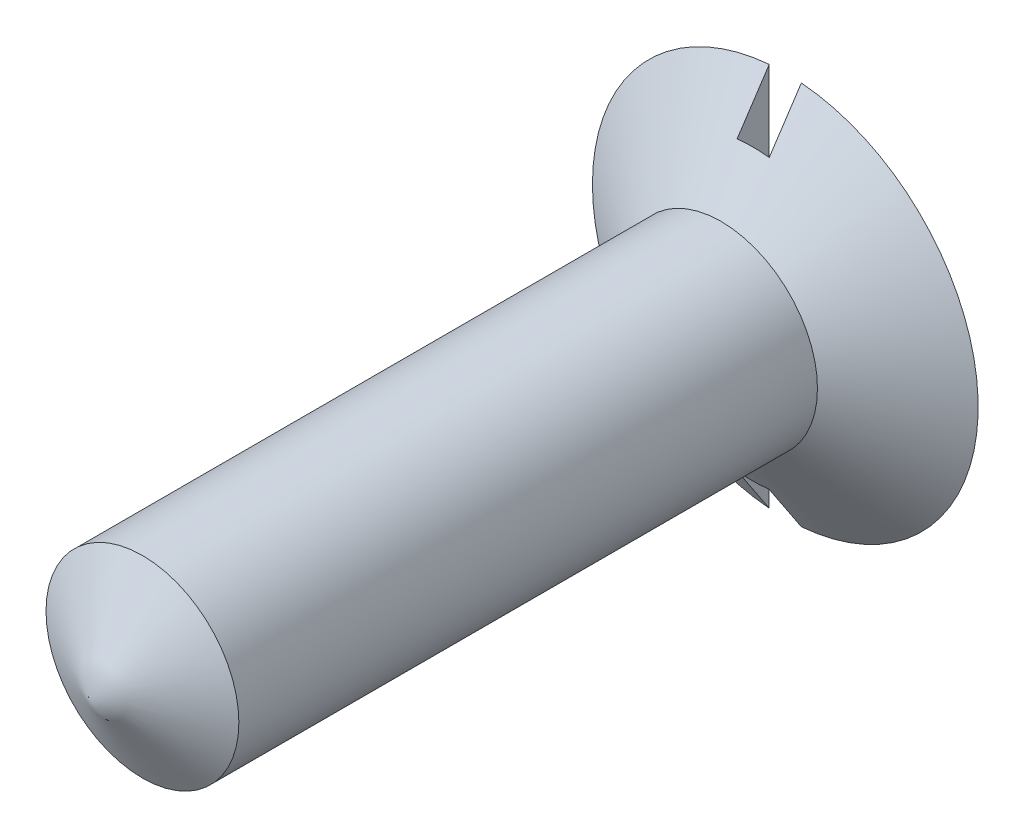
from build123d import *

# Parameters (mm, degrees)
SKETCH1_W          = 4.5
SKETCH1_H          = 27
CUT_EXTRUDE1_DEPTH = 15


with BuildPart() as part:
    # Sketch1 → Revolve3 (revolve)
    with BuildSketch(Plane(origin=(0, 0, 0), x_dir=(1, 0, 0), z_dir=(0, 1, 0)), mode=Mode.PRIVATE) as revolve3_sk:
        with Locations((2.25, 0)):
            Rectangle(SKETCH1_W, SKETCH1_H)
        Polygon((0, -13.5), (4.5, -13.5), (0, -16), align=None)
        Polygon((9, 16.5), (4.5, 13.5), (0, 13.5), (0, 16.5), align=None)
    revolve(revolve3_sk.sketch.rotate(Axis((0, 0, -13.5), (0, 0, 1)), 180), axis=Axis((0, 0, -13.5), (0, 0, 1)))

    # Sketch2 → Cut-Extrude1 (cut, symmetric)
    with BuildSketch(Plane(origin=(0, 0, 0), x_dir=(1, 0, 0), z_dir=(0, 1, 0))):
        Polygon((0, 16.5), (0.75, 16.5), (0.75, 15), (-0.75, 15), (-0.75, 16.5), align=None)
    extrude(amount=CUT_EXTRUDE1_DEPTH, both=True, mode=Mode.SUBTRACT)


solid = part.part
